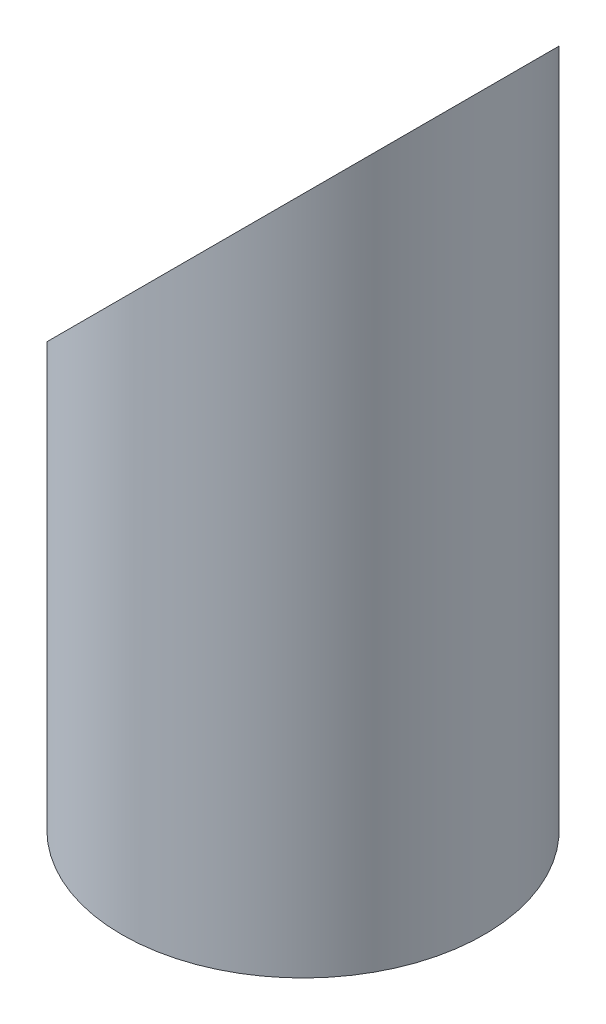
SolidWorks part; units mm, degrees
material "STKM13A"
ref_plane "Front Plane" through (0, 0, 0) normal (0, 0, 1) x (1, 0, 0)
ref_plane "Top Plane" through (0, 0, 0) normal (0, 1, 0) x (1, 0, 0)
ref_plane "Right Plane" through (0, 0, 0) normal (1, 0, 0) x (0, 0, -1)
sketch "Sketch1" plane through (0, 0, 0) normal (0, 1, 0) x (1, 0, 0)
  circle A0 centre (0, 0) radius 19.05
  circle A1 centre (0, 0) radius 17.05
  dimension "D1" = 38.1
  dimension "D2" = 2
extrude "Boss-Extrude1" add sketch "Sketch1" along normal blind 77
sketch "Sketch2" plane through (0, 0, 0) normal (0, 0, 1) x (1, 0, 0)
  line L0 (19.05, 77) -> (-19.05, 38.9)
  line L1 (-19.05, 77) -> (-19.05, 0) construction
  line L2 (-19.05, 38.9) -> (-19.05, 77)
  line L3 (-19.05, 77) -> (19.05, 77)
  dimension "D1" = 45
extrude "Cut-Extrude1" cut sketch "Sketch2" against normal through all both and the other way through all
